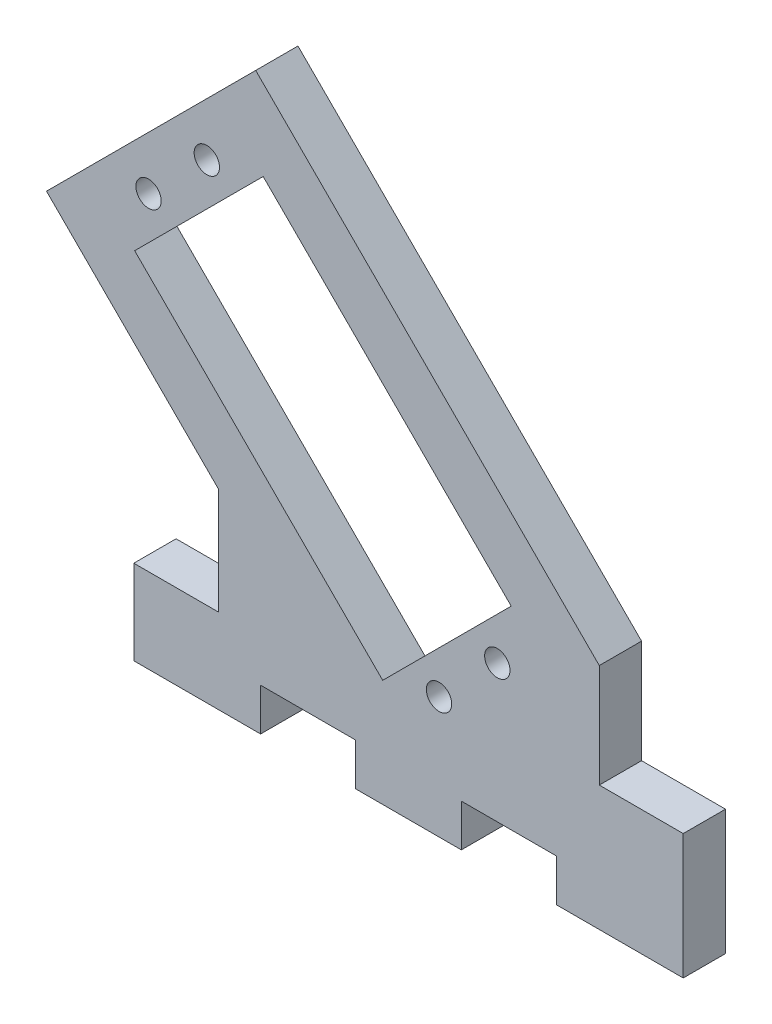
SolidWorks part; units mm, degrees
ref_plane "前视基准面" through (0, 0, 0) normal (0, 0, 1) x (1, 0, 0)
ref_plane "上视基准面" through (0, 0, 0) normal (0, 1, 0) x (1, 0, 0)
ref_plane "右视基准面" through (0, 0, 0) normal (1, 0, 0) x (0, 0, -1)
other "Configuration Table"
sketch "草图1" plane through (0, 0, 0) normal (0, 0, 1) x (1, 0, 0)
  line L0 (-12.6486, -34.7078) -> (-27.6486, -34.7078)
  line L1 (-27.6486, -34.7078) -> (-27.6486, -24.7078)
  line L2 (-27.6486, -24.7078) -> (-17.6486, -24.7078)
  line L3 (-17.6486, -24.7078) -> (-17.6486, -12.0858)
  line L4 (-17.6486, -12.0858) -> (-37.9779, 8.2435)
  line L5 (-37.9779, 8.2435) -> (-13.2292, 32.9922)
  line L6 (-13.2292, 32.9922) -> (27.4208, -7.6578)
  line L7 (27.4208, -7.6578) -> (27.4208, -19.9078)
  line L8 (27.4208, -19.9078) -> (37.3514, -19.9078)
  line L9 (37.3514, -19.9078) -> (37.3514, -34.7078)
  line L10 (37.3514, -34.7078) -> (22.3514, -34.7078)
  line L11 (22.3514, -34.7078) -> (22.3514, -29.7078)
  line L12 (22.3514, -29.7078) -> (11.1014, -29.7078)
  line L13 (11.1014, -29.7078) -> (11.1014, -34.7078)
  line L14 (11.1014, -34.7078) -> (-1.3986, -34.7078)
  line L15 (-1.3986, -34.7078) -> (-1.3986, -29.7078)
  line L16 (-1.3986, -29.7078) -> (-12.6486, -29.7078)
  line L17 (-12.6486, -29.7078) -> (-12.6486, -34.7078)
  line L18 (-27.5481, 7.3596) -> (1.7968, -21.9853)
  line L19 (1.7968, -21.9853) -> (16.9996, -6.7825)
  line L20 (16.9996, -6.7825) -> (-12.3453, 22.5624)
  line L21 (-12.3453, 22.5624) -> (-27.5481, 7.3596)
  line L22 (-25.9041, 14.0241) -> (-19.0098, 20.9184)
  circle A0 centre (-19.0098, 20.9184) radius 1.5
  circle A1 centre (-25.9041, 14.0241) radius 1.5
  circle A2 centre (15.3556, -13.447) radius 1.5
  circle A3 centre (8.4613, -20.3413) radius 1.5
  point P21 (-1.3986, -32.2078)
  dimension "D20" = 3
  dimension "D1" = 65
  dimension "D2" = 12.5
  dimension "D3" = 11.25
  dimension "D4" = 5
  dimension "D5" = 5
  dimension "D6" = 5
  dimension "D7" = 10
  dimension "D8" = 10
  dimension "D9" = 67.7
  dimension "D10" = 35
  dimension "D11" = 12.25
  dimension "D12" = 14.8
  dimension "D13" = 15
  dimension "D14" = 45
  dimension "D15" = 21.5
  dimension "D16" = 41.5
  dimension "D17" = 6.75
  dimension "D18" = 8
  dimension "D19" = 11.25
  dimension "D21" = 9.75
  dimension "D22" = 48.6
extrude "凸台-拉伸1" add sketch "草图1" along normal blind 5
